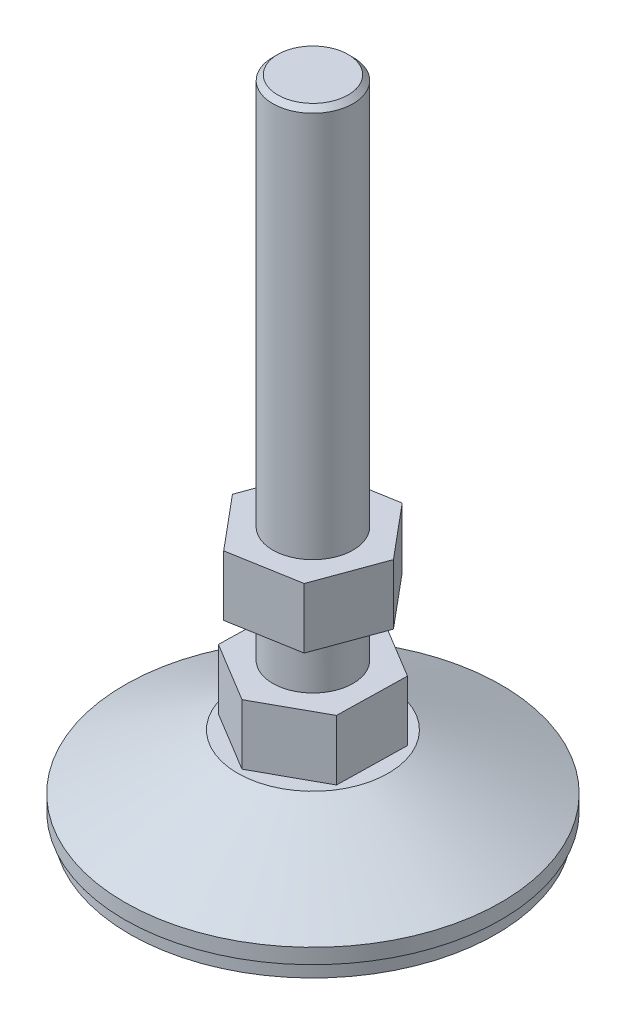
SolidWorks part; units mm, degrees
ref_plane "Front Plane" through (0, 0, 0) normal (0, 0, 1) x (1, 0, 0)
ref_plane "Top Plane" through (0, 0, 0) normal (0, 1, 0) x (1, 0, 0)
ref_plane "Right Plane" through (0, 0, 0) normal (1, 0, 0) x (0, 0, -1)
sketch "Sketch1" plane through (0, 0, 0) normal (0, 0, 1) x (1, 0, 0)
  line L0 (0, 0) -> (0, -50000) construction
  line L1 (-37.5, 10.3727) -> (-15, 21.3727)
  line L2 (0, 134.3727) -> (-8, 134.3727)
  line L3 (0, 134.3727) -> (0, 4.3727)
  line L4 (-15, 21.3727) -> (-8, 21.3727)
  line L5 (-8, 134.3727) -> (-8, 21.3727)
  line L6 (-37.5, 10.3727) -> (-37.5, 7.3727)
  line L7 (-37.5, 7.3727) -> (-36.5, 7.3727)
  line L8 (-36.5, 7.3727) -> (-36.5, 4.3727)
  line L9 (-36.5, 4.3727) -> (0, 4.3727)
  dimension "D1" = 130
  dimension "D2" = 8
  dimension "D3" = 14
  dimension "D4" = 3
  dimension "D5" = 1
  dimension "D6" = 15
  dimension "D7" = 37.5
  dimension "D8" = 3
revolve "Revolve1" add sketch "Sketch1" angle 360 about L0
cosmetic thread "Cosmetic Thread1" parameters "D2"=10.5
cosmetic thread "Cosmetic Thread2" parameters "D2"=10.5
sketch "Sketch2" plane through (0, 21.3727, 0) normal (0, 1, 0) x (-1, 0, 0)
  line L1 (-11.8593, 7.1663) -> (-12.1359, -6.6873)
  line L2 (-12.1359, -6.6873) -> (-0.2766, -13.8536)
  line L3 (-0.2766, -13.8536) -> (11.8593, -7.1663)
  line L4 (11.8593, -7.1663) -> (12.1359, 6.6873)
  line L5 (12.1359, 6.6873) -> (0.2766, 13.8536)
  line L6 (0.2766, 13.8536) -> (-11.8593, 7.1663)
  circle A0 centre (0, 0) radius 12 construction
  dimension "D1" = 24
extrude "Extrude1" add sketch "Sketch2" along normal blind 12
sketch "Sketch3" plane through (0, 21.3727, 0) normal (0, 1, 0) x (-1, 0, 0)
  line L1 (-8.8878, 10.6305) -> (-13.6502, -2.3818)
  line L2 (-13.6502, -2.3818) -> (-4.7624, -13.0123)
  line L3 (-4.7624, -13.0123) -> (8.8878, -10.6305)
  line L4 (8.8878, -10.6305) -> (13.6502, 2.3818)
  line L5 (13.6502, 2.3818) -> (4.7624, 13.0123)
  line L6 (4.7624, 13.0123) -> (-8.8878, 10.6305)
  circle A0 centre (0, 0) radius 12 construction
  dimension "D1" = 24
extrude "Extrude2" add sketch "Sketch3" against normal blind 12 from offset 35
chamfer "Chamfer1" distance 1 angle 45 1 edges at (0, 134.3727, 8)
